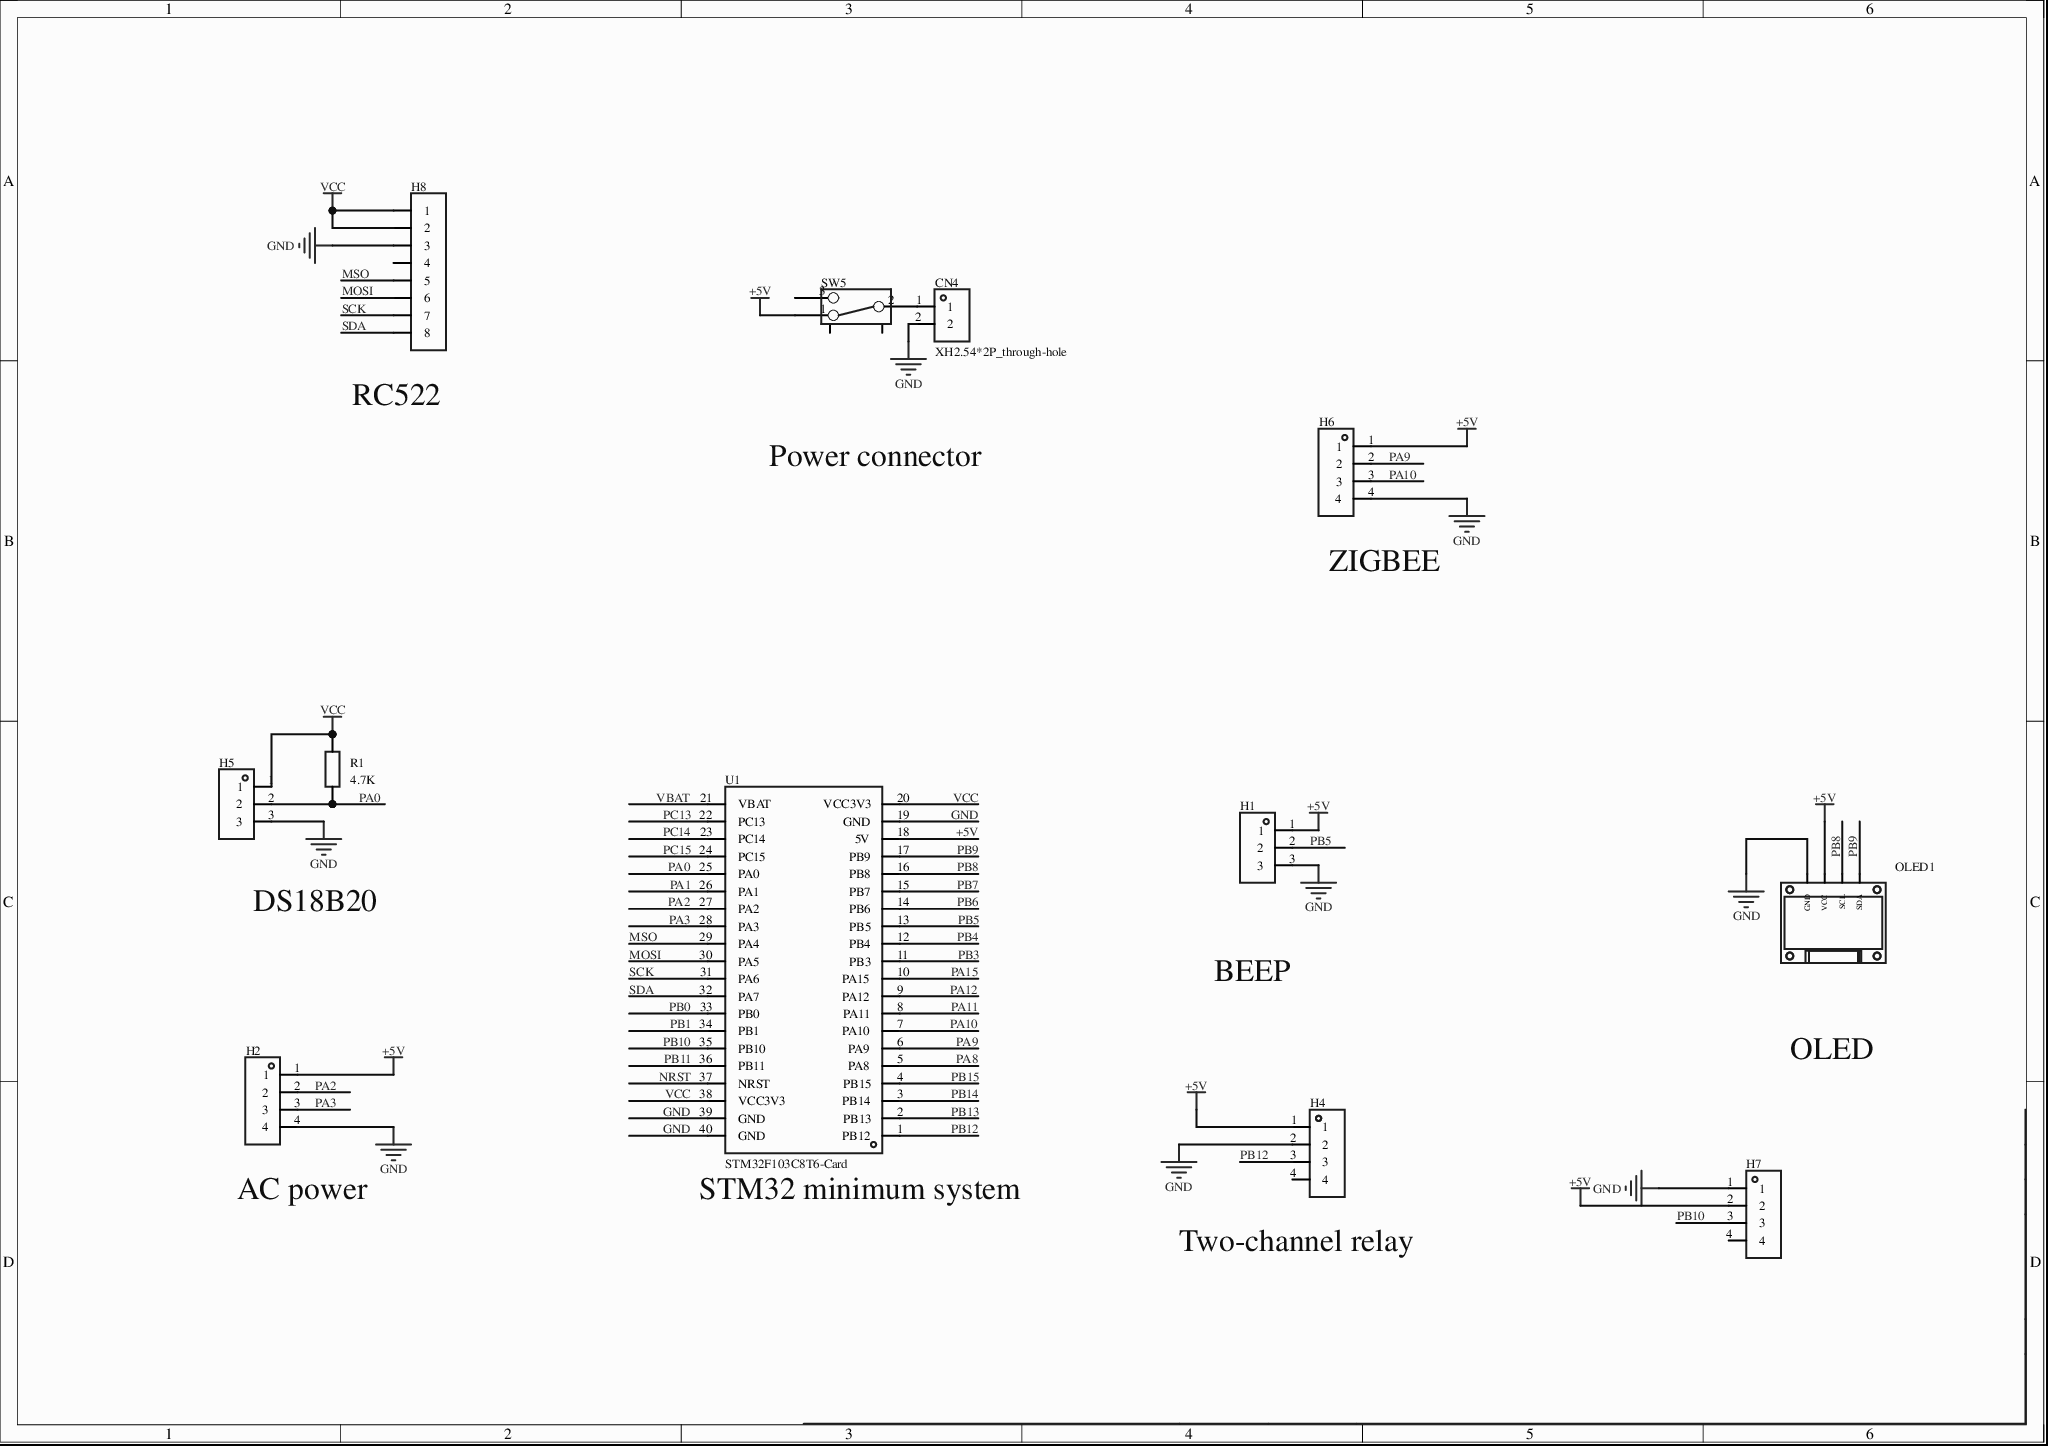
[diagram p0: MISC88997-3.schdoc]
# Altium project MISC88997-2.PrjPcb
1 sheet, 12 parts. Net scope: global (net labels, ports and power ports of the same name join across sheets).
Board file: MISC88997.pcbdoc

## Sheet MISC88997-3.schdoc
size 297 x 209 mm; Version: V1.0; @Project Name: MISC88997; @Page Count: 1; @Update Date: 2026-04-07; @Create Date: 2026-04-07; @Schematic Name: MISC88997; @Page No: 1; @Create Time: 23:22:16; @Update Time: 17:32:40; @Board Name: MISC88997

### Parts
CN4  XH2.54*2P_through-hole  [CONN-TH_2P-P2.50-XH2.54-2P]
H1  (no value)  [HDR-TH_3P-P2.54-V-F]
H2  (no value)  [HDR-TH_4P-P2.54-V-F]
H4  (no value)  [HDR-TH_4P-P2.54-V-F]
H5  (no value)  [HDR-TH_3P-P2.54-V-F]
H6  (no value)  [HDR-TH_4P-P2.54-V-F]
H7  (no value)  [HDR-TH_4P-P2.54-V-M]
H8  (no value)  [HDR-TH_8P-P2.54-V-F-1]
OLED1  (no value)  [0.96OLED_4P]
R1  4.7K  [R0603]
SW5  (no value)  [拨动开关]
U1  STM32F103C8T6-Card  [CONN-TH_L53.3-W22.9_STM32F103C8T6-CARD]

### Nets
+5V: H1.1 H2.1 H4.1 H6.1 H7.2 OLED1.2(VCC) SW5.1 U1.18(5V)
GND: CN4.2 H1.3 H2.4 H4.2 H5.3 H6.4 H7.1 H8.3 OLED1.1(GND) U1.19(GND) U1.39(GND) U1.40(GND)
VCC: H5.1 H8.1 H8.2 R1.2 U1.20(VCC3V3) U1.38(VCC3V3)
MOSI: H8.6 U1.30(PA5)
MSO: H8.5 U1.29(PA4)
NRST: U1.37(NRST)
PA0: H5.2 R1.1 U1.25(PA0)
PA1: U1.26(PA1)
PA2: H2.2 U1.27(PA2)
PA3: H2.3 U1.28(PA3)
PA8: U1.5(PA8)
PA9: H6.2 U1.6(PA9)
PA10: H6.3 U1.7(PA10)
PA11: U1.8(PA11)
PA12: U1.9(PA12)
PA15: U1.10(PA15)
PB0: U1.33(PB0)
PB1: U1.34(PB1)
PB3: U1.11(PB3)
PB4: U1.12(PB4)
PB5: H1.2 U1.13(PB5)
PB6: U1.14(PB6)
PB7: U1.15(PB7)
PB8: OLED1.3(SCL) U1.16(PB8)
PB9: OLED1.4(SDA) U1.17(PB9)
PB10: H7.3 U1.35(PB10)
PB11: U1.36(PB11)
PB12: H4.3 U1.1(PB12)
PB13: U1.2(PB13)
PB14: U1.3(PB14)
PB15: U1.4(PB15)
PC13: U1.22(PC13)
PC14: U1.23(PC14)
PC15: U1.24(PC15)
SCK: H8.7 U1.31(PA6)
SDA: H8.8 U1.32(PA7)
VBAT: U1.21(VBAT)
NetCN4_1: CN4.1 SW5.2

Not connected (* = marked no-connect by the designer): H4 4; H7 4; H8 4; SW5 3 4 5

### Notes on the sheet
- (near H8) RC522
- Power connector
- (near H6) ZIGBEE
- DS18B20
- BEEP
- OLED
- (near H2) AC power
- (near U1) STM32 minimum system
- (near H4) Two-channel relay

### Library data of the parts
CN4 = XH2.54*2P_直插: 3D Model: 325c595e30db4df8abe76612dd40b0fa0819f05c4eef4c71ace90d822a990e87; 3D Model Transform: 295.275,228.346,0,180,0,0,-0.002,-20.079,-137.795; AddInBom: yes; Device: XH2.54*2P_through-hole; Symbol: XH2.54*2P_through-hole; LCSC Part Name: XH2.54*2P_直插; Supplier Part: C9900008615; Manufacturer Part: XH2.54*2P_直插; Supplier Footprint: XH2.54_2P; JLCPCB Part Class: Extended Part; Supplier: LCSC; FootprintName: CONN-TH_2P-P2.50-XH2.54-2P; ConvertToPcb: yes; ModelName: CONN-TH_2P-P2.50-XH2.54-2P
H1 H5 = HDR-F_2.54_1x3P: Symbol: PM254V-11-03-H85; 3D Model: f3b3cc5aae9641bf9e56fc160cef875b; 3D Model Transform: 299.9994,100,0,0,0,0,0,0,-118.11; ConvertToPcb: yes; ModelName: HDR2.54-F-LI-1X3P; Device: HDR-F_2.54_1x3P; Supplier Part: C541850; Supplier Footprint: 插件; FootprintName: HDR-TH_3P-P2.54-V-F; AddInBom: yes
H2 H4 = HDR-F_2.54_1x4P: Symbol: 2.54-1*4P female; ConvertToPcb: yes; ModelId: d187812051054f85879fcaa51a310d8e0819f05c4eef4c71ace90d822a990e87; ModelTransform: 419.6842,98.464,0,0,0,0,0,0,-118.11; Device: HDR-F_2.54_1x4P; FootprintName: HDR-TH_4P-P2.54-V-F; AddInBom: yes; SupplierPart: C2718488; Supplier Footprint: 插件; ModelName: HDR-TH_4P-P2.54-V-F
H6 = HDR-F_2.54_1x4P: Symbol: 2.54-1*4P female; 3D Model: d187812051054f85879fcaa51a310d8e0819f05c4eef4c71ace90d822a990e87; 3D Model Transform: 419.6842,98.464,0,0,0,0,0,0,-118.11; ConvertToPcb: yes; Device: HDR-F_2.54_1x4P; Supplier Part: C2718488; Supplier Footprint: 插件; FootprintName: HDR-TH_4P-P2.54-V-F; AddInBom: yes; ModelName: HDR-TH_4P-P2.54-V-F
H7 = HDR-M_2.54_1x4P: Symbol: PZ254V-11-04P; ConvertToPcb: yes; ModelId: 112f4d05e8d64e99ab9a333894bea4f90819f05c4eef4c71ace90d822a990e87; ModelName: HDR-TH_4P-P2.54-M-LI-1X4P; ModelTransform: 399.999,104.7242,0,0,0,0,0,0,-118.11; Device: HDR-M_2.54_1x4P; AddInBom: yes; SupplierPart: C492403; Supplier Footprint: 插件; FootprintName: HDR-TH_4P-P2.54-V-M
H8 = HDR-F_2.54_1x8P: Symbol: Header-Female-2.54_1x8; AddInBom: yes; ModelId: 0f7e4d9227ef4fa08d5469c22cc70cdb; ModelName: HDR-F-2.54_1x8; ModelTransform: 799.99844,100,0,0,0,0,0,0,-118.11; Device: HDR-F_2.54_1x8P; ConvertToPcb: yes; FootprintName: HDR-TH_8P-P2.54-V-F-1; SupplierPart: C27438; Supplier Footprint: 插件
OLED1 = 0.96OLED模块_4P: Device: 0.96OLED module_4P; ConvertToPcb: yes; ModelId: 79c000fdb68d45a296c2e9bedf4f9055; ModelTransform: 1393.69792,1318.895,0,0,0,0,0,-560.079,-137.795; Symbol: 0.96OLED module_4P; FootprintName: 0.96OLED_4P; AddInBom: yes; Supplier Footprint: 插件; ModelName: 0.96OLED_4P
R1 = Res_0603: Symbol: resistor; 3D Model: fc143cca1e79419f9cd78b61e9279f080819f05c4eef4c71ace90d822a990e87; 3D Model Transform: 31.8897,63.7794,0,90,0,0,0,0,0; ConvertToPcb: yes; Device: Res_0603; Supplier Footprint: 0603; Value: 4.7K; AddInBom: yes; FootprintName: R0603; ModelName: R0603
SW5 = 拨动开关_正: Device: toggle switch_positive; Symbol: toggle switch; ConvertToPcb: yes; ModelId: 4321fe59a4074cbfb4989553f297c68f0819f05c4eef4c71ace90d822a990e87; ModelName: SW-TH_SS-12D02-VG4; ModelTransform: 370.09,208.7,472.35,0,0,0,0,0,-110; FootprintName: toggle switch; AddInBom: yes; Supplier Footprint: 插件
U1 = STM32F103C8T6-Card: AddInBom: yes; Device: STM32F103C8T6-Card; Symbol: STM32F103C8T6-CARD; FootprintName: CONN-TH_L53.3-W22.9_STM32F103C8T6-CARD; LCSC Part Name: STM32F103C8T6-Card; SupplierPart: C9900077949; ManufacturerPart: STM32F103C8T6-Card; Supplier Footprint: 插件; Supplier: LCSC; ConvertToPcb: yes